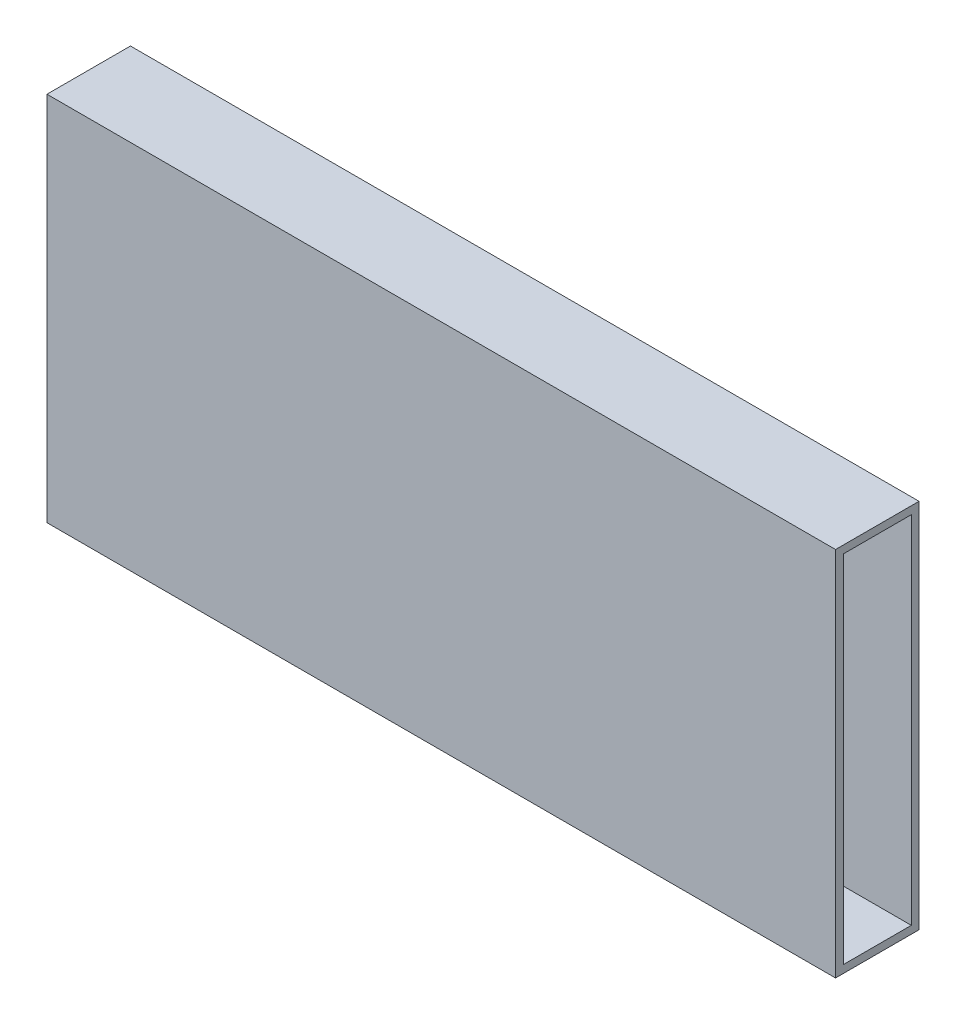
SolidWorks part; units mm, degrees
ref_plane "Front Plane" through (0, 0, 0) normal (0, 0, 1) x (1, 0, 0)
ref_plane "Top Plane" through (0, 0, 0) normal (0, 1, 0) x (1, 0, 0)
ref_plane "Right Plane" through (0, 0, 0) normal (1, 0, 0) x (0, 0, -1)
sketch "Sketch1" plane through (0, 0, 0) normal (0, 0, 1) x (1, 0, 0)
  line L1 (-510, 240) -> (510, 240)
  line L2 (-510, 240) -> (-510, -240)
  line L3 (-510, -240) -> (510, -240)
  line L4 (510, 240) -> (510, -240)
  line L5 (-510, 240) -> (510, -240) construction
  line L6 (-510, -240) -> (510, 240) construction
  point P0 (0, 0)
  dimension "D1" = 1020
  dimension "D2" = 480
extrude "Boss-Extrude1" add sketch "Sketch1" along normal blind 108
shell "Shell1" thickness 10
sketch "Sketch2" plane through (0, 0, 0) normal (0, 0, -1) x (-1, 0, 0)
  circle A0 centre (-397.4709, 192.1875) radius 18.75
  circle A1 centre (-395.5331, -192.1875) radius 18.75
  circle A2 centre (465.0919, -191.8371) radius 18.75
  circle A3 centre (465.0919, 191.8371) radius 18.75
extrude "Cut-Extrude1" cut sketch "Sketch2" against normal blind 10
